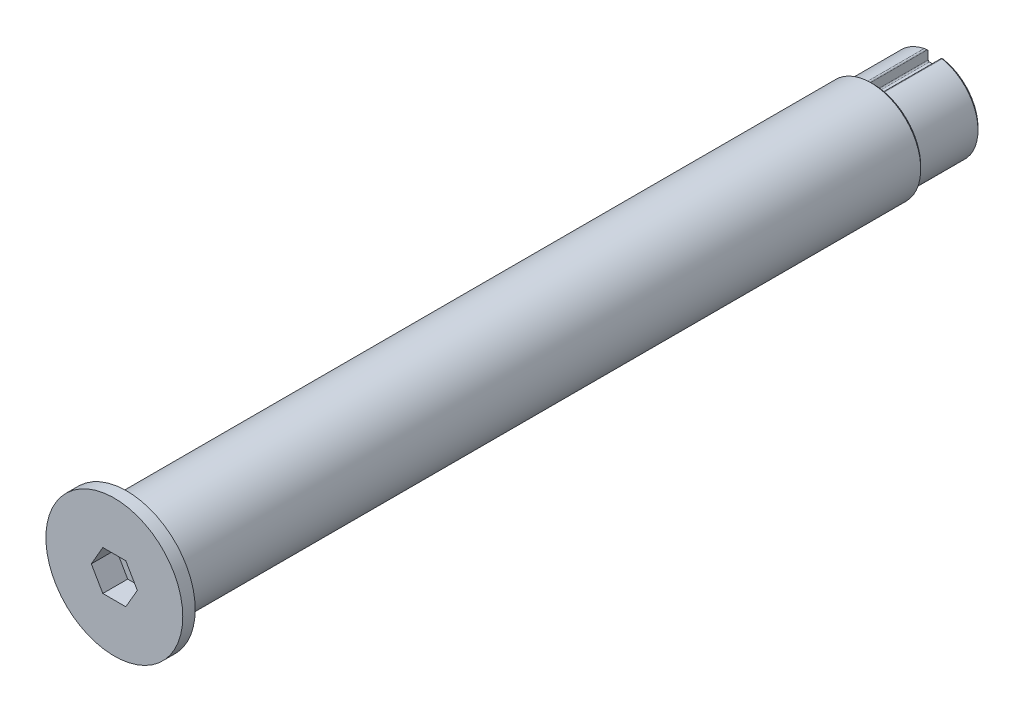
from build123d import *

# Parameters (mm, degrees)
SKETCH_1_R          = 20
EXTRUDE_1_DEPTH     = 325
SKETCH_2_R          = 27.5
EXTRUDE_2_DEPTH     = 5
CUT_EXTRUDE_1_DEPTH = 10
SKETCH_4_OUTSIDE_W  = 124.808
SKETCH_4_OUTSIDE_H  = 124.808
SKETCH_4_OUTSIDE_R  = 18
CUT_EXTRUDE_2_DEPTH = 25
CHAMFER_1_SIZE      = 1
CHAMFER_2_SIZE      = 1
FILLET_1_R          = 0.5
SKETCH_5_W          = 6
SKETCH_5_H          = 10
CUT_EXTRUDE_3_DEPTH = 25
FILLET_2_R          = 0.5


with BuildPart() as part:
    # 草图1 → 凸台-拉伸1 (new body)
    with BuildSketch(Plane.XY):
        Circle(SKETCH_1_R)
    extrude(amount=EXTRUDE_1_DEPTH)

    # 草图2 → 凸台-拉伸2 (add)
    with BuildSketch(Plane.XY.offset(325)):
        Circle(SKETCH_2_R)
    extrude(amount=EXTRUDE_2_DEPTH)

    # 草图3 → 切除-拉伸1 (cut)
    with BuildSketch(Plane.XY.offset(330)):
        Polygon((9.237604307, 0), (4.618802154, 8), (-4.618802154, 8), (-9.237604307, 0), (-4.618802154, -8), (4.618802154, -8), align=None)
    extrude(amount=-CUT_EXTRUDE_1_DEPTH, mode=Mode.SUBTRACT)

    # 草图4 outside → 切除-拉伸2 (cut)
    with BuildSketch(Plane(origin=(0, 0, 0), x_dir=(-1, 0, 0), z_dir=(0, 0, -1))):
        Rectangle(SKETCH_4_OUTSIDE_W, SKETCH_4_OUTSIDE_H)
        Circle(SKETCH_4_OUTSIDE_R, mode=Mode.SUBTRACT)
    extrude(amount=-CUT_EXTRUDE_2_DEPTH, mode=Mode.SUBTRACT)

    # 倒角1
    chamfer_1_edges = [part.edges().sort_by_distance(p)[0] for p in [
        (-20, 0, 25),
    ]]
    chamfer(chamfer_1_edges, length=CHAMFER_1_SIZE)

    # 倒角2
    chamfer_2_edges = [part.edges().sort_by_distance(p)[0] for p in [
        (18, 0, 0),
    ]]
    chamfer(chamfer_2_edges, length=CHAMFER_2_SIZE)

    # 圆角1
    fillet_1_edges = [part.edges().sort_by_distance(p)[0] for p in [
        (-20, 0, 325),
    ]]
    fillet(fillet_1_edges, radius=FILLET_1_R)

    # 草图5 → 切除-拉伸3 (cut)
    with BuildSketch(Plane(origin=(0, 0, 0), x_dir=(-1, 0, 0), z_dir=(0, 0, -1))):
        with Locations((0, 18)):
            Rectangle(SKETCH_5_W, SKETCH_5_H)
    extrude(amount=-CUT_EXTRUDE_3_DEPTH, mode=Mode.SUBTRACT)

    # 圆角2
    fillet_2_edges = [part.edges().sort_by_distance(p)[0] for p in [
        (-3, 13, 12.5),
        (3, 13, 12.5),
        (3, 17.748239349, 13),
        (-3, 17.748239349, 13),
    ]]
    fillet(fillet_2_edges, radius=FILLET_2_R)


solid = part.part
